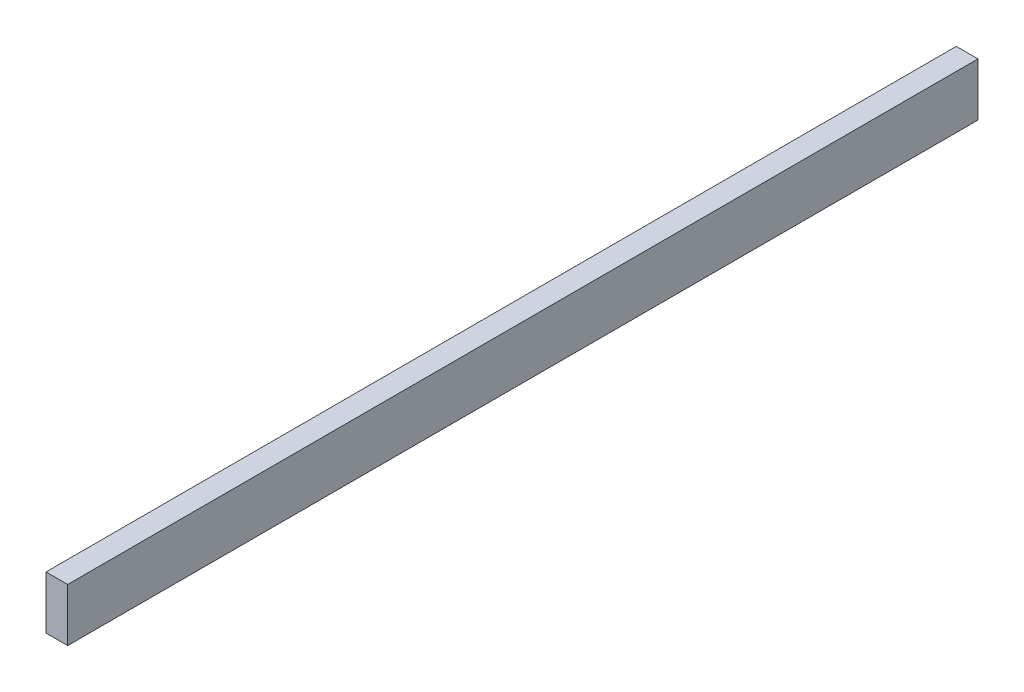
from build123d import *

# Parameters (mm, degrees)
SKETCH1_W           = 1890
SKETCH1_H           = 110
BOSS_EXTRUDE1_DEPTH = 22.5


with BuildPart() as part:
    # Sketch1 → Boss-Extrude1 (new, symmetric)
    with BuildSketch(Plane(origin=(0, 0, 0), x_dir=(0, 0, -1), z_dir=(1, 0, 0))):
        Rectangle(SKETCH1_W, SKETCH1_H)
    extrude(amount=BOSS_EXTRUDE1_DEPTH, both=True)


solid = part.part
